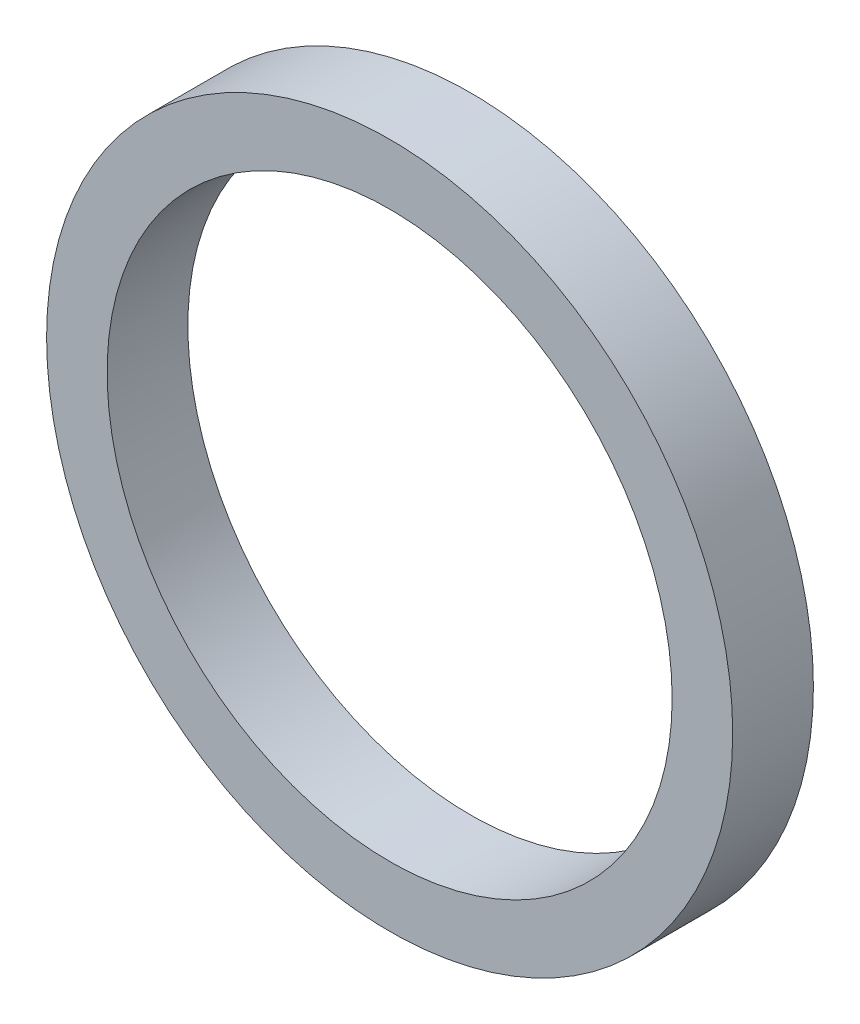
from build123d import *

# Parameters (mm, degrees)
SKETCH_1_R      = 21.25
SKETCH_1_R_2    = 17.5
EXTRUDE_1_DEPTH = 5


with BuildPart() as part:
    # 草图1 → 凸台-拉伸1 (new body)
    with BuildSketch(Plane.XY):
        Circle(SKETCH_1_R)
        Circle(SKETCH_1_R_2, mode=Mode.SUBTRACT)
    extrude(amount=EXTRUDE_1_DEPTH)


solid = part.part
